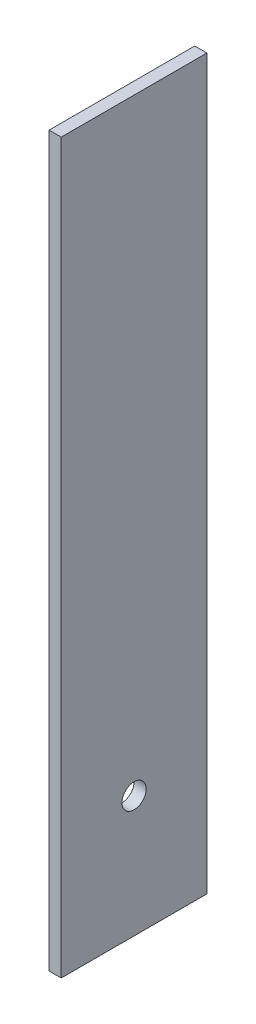
SolidWorks part; units mm, degrees
ref_plane "前视基准面" through (0, 0, 0) normal (0, 0, 1) x (1, 0, 0)
ref_plane "上视基准面" through (0, 0, 0) normal (0, 1, 0) x (1, 0, 0)
ref_plane "右视基准面" through (0, 0, 0) normal (1, 0, 0) x (0, 0, -1)
sketch "草图1" plane through (0, 0, 0) normal (0, 0, 1) x (1, 0, 0)
  line L1 (-2.5, -150) -> (2.5, -150)
  line L2 (-2.5, -150) -> (-2.5, 150)
  line L3 (-2.5, 150) -> (2.5, 150)
  line L4 (2.5, -150) -> (2.5, 150)
  line L5 (-2.5, -150) -> (2.5, 150) construction
  line L6 (-2.5, 150) -> (2.5, -150) construction
  point P0 (0, 0)
  dimension "D1" = 300
  dimension "D2" = 5
extrude "凸台-拉伸1" add sketch "草图1" along normal blind 60
sketch "草图2" plane through (2.5, 0, 0) normal (1, 0, 0) x (0, 0, -1)
  line L0 (-60, -150) -> (0, -150) construction
  line L1 (0, -150) -> (0, 150) construction
  circle A0 centre (-30, -100) radius 5
  dimension "D1" = 10
  dimension "D2" = 50
  dimension "D3" = 30
extrude "切除-拉伸1" cut sketch "草图2" against normal blind 20
ref_plane "基准面1" through (0, 0, 30) normal (0, 0, 1) x (1, 0, 0)
